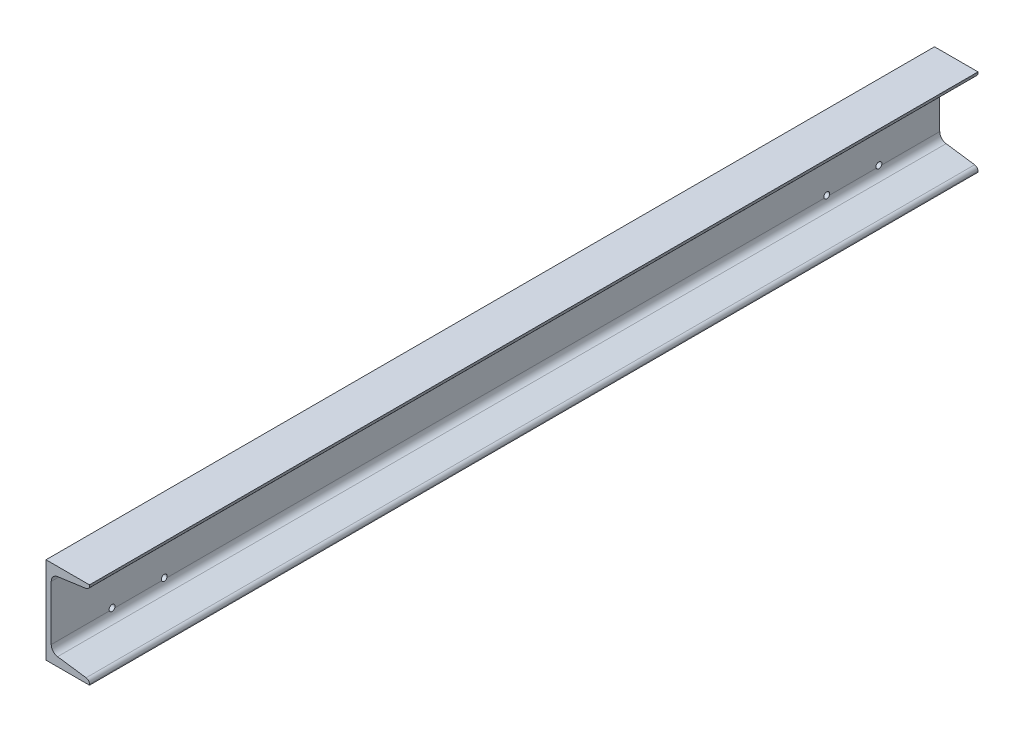
SolidWorks part; units mm, degrees
material "1023 碳钢板 (SS)"
ref_plane "Front Plane" through (0, 0, 0) normal (0, 0, 1) x (1, 0, 0)
ref_plane "Top Plane" through (0, 0, 0) normal (0, 1, 0) x (1, 0, 0)
ref_plane "Right Plane" through (0, 0, 0) normal (1, 0, 0) x (0, 0, -1)
sketch "Sketch1" plane through (0, 0, 0) normal (0, 0, 1) x (1, 0, 0)
  line L0 (0, 0) -> (-50, 0)
  line L1 (-50, 0) -> (-50, -100)
  line L2 (-50, -100) -> (0, -100)
  line L3 (0, -100) -> (0, -98.9253)
  line L4 (-3.8737, -94.4691) -> (-36.683, -89.8581)
  line L5 (-44, -81.4408) -> (-44, -18.5592)
  line L6 (-36.683, -10.1419) -> (-3.8737, -5.5309)
  line L7 (0, -1.0747) -> (0, 0)
  line L8 (-25, -100) -> (-25, -91.5) construction
  arc A0 (-36.683, -89.8581) -> (-44, -81.4408) centre (-35.5, -81.4408) cw
  arc A1 (-44, -18.5592) -> (-36.683, -10.1419) centre (-35.5, -18.5592) cw
  arc A2 (0, -98.9253) -> (-3.8737, -94.4691) centre (-4.5, -98.9253) ccw
  arc A3 (-3.8737, -5.5309) -> (0, -1.0747) centre (-4.5, -1.0747) ccw
  dimension "D8" = 8.5
  dimension "D9" = 4.5
  dimension "D1" = 100
  dimension "D2" = 8
  dimension "D3" = 8
  dimension "D4" = 50
  dimension "D5" = 6
  dimension "D6" = 25
  dimension "D7" = 8.5
extrude "Boss-Extrude1" add sketch "Sketch1" along normal blind 1022
sketch "Sketch2" plane through (-50, 0, 0) normal (-1, 0, 0) x (0, 0, 1)
  line L0 (0, 0) -> (0, -100) construction
  line L1 (70, -80) -> (130, -80) construction
  line L2 (70, -80) -> (70, -20) construction
  line L3 (70, -20) -> (130, -20) construction
  line L4 (130, -80) -> (130, -20) construction
  line L5 (70, -80) -> (130, -20) construction
  line L6 (70, -20) -> (130, -80) construction
  line L7 (1022, 0) -> (0, 0) construction
  circle A0 centre (70, -20) radius 3
  circle A1 centre (130, -20) radius 3
  circle A2 centre (130, -80) radius 3
  circle A3 centre (70, -80) radius 3
  circle A4 centre (892, -20) radius 3
  circle A5 centre (952, -20) radius 3
  circle A6 centre (952, -80) radius 3
  circle A7 centre (892, -80) radius 3
  point P0 (100, -50)
  dimension "D5" = 6
  dimension "D1" = 60
  dimension "D2" = 60
  dimension "D3" = 70
  dimension "D4" = 20
  dimension "D6" = 2
hole_wizard "M8 Tapped Hole1" positions "Sketch3" profile "Sketch4" tap size "M8" standard "ISO"
sketch "Sketch3" plane through (-50, 0, 0) normal (-1, 0, 0) x (0, 0, 1)
  point P0 (70, -20)
  point P3 (130, -20)
  point P6 (130, -80)
  point P9 (70, -80)
  point P12 (892, -20)
  point P15 (952, -20)
  point P18 (952, -80)
  point P21 (892, -80)
sketch "Sketch4" plane through (-50, -20, 70) normal (0, 1, 0) x (0, 0, 1)
  line L0 (0, 0) -> (0, 21.7929)
  line L1 (0, 21.7929) -> (3.4, 19.75)
  line L2 (3.4, 19.75) -> (3.4, 0)
  line L5 (3.4, 0) -> (0, 0)
  line L10 (0, 21.7929) -> (-3.4, 19.75) construction
  line L11 (0, -6.35) -> (0, 107.95) construction
  dimension "螺纹孔钻头直径" = 6.8
  dimension "螺纹孔钻头深度" = 19.75
  dimension "导头角度" = 118
cosmetic thread "Hole thread line 1"
cosmetic thread "Hole thread line 2"
cosmetic thread "Hole thread line 3"
cosmetic thread "Hole thread line 4"
cosmetic thread "Hole thread line 5"
cosmetic thread "Hole thread line 6"
cosmetic thread "Hole thread line 7"
cosmetic thread "Hole thread line 8"
